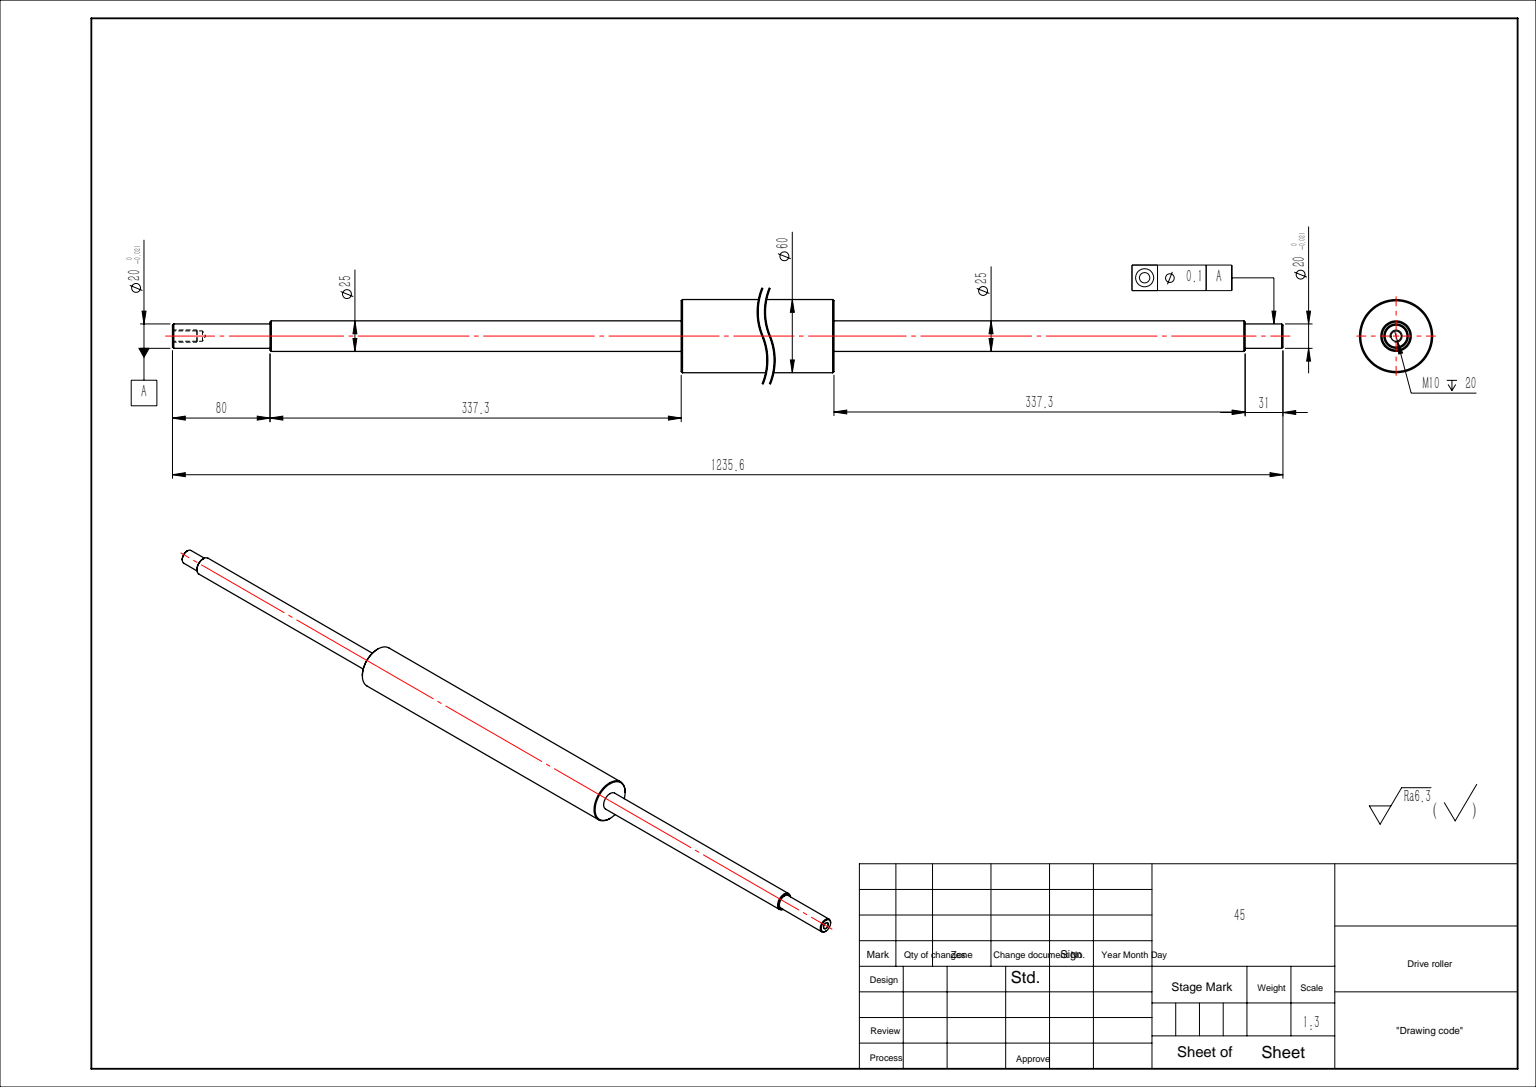
SolidWorks part; units mm, degrees
material "45"
ref_plane "前视基准面" through (0, 0, 0) normal (0, 0, 1) x (1, 0, 0)
ref_plane "上视基准面" through (0, 0, 0) normal (0, 1, 0) x (1, 0, 0)
ref_plane "右视基准面" through (0, 0, 0) normal (1, 0, 0) x (0, 0, -1)
sketch "草图1" plane through (0, 0, 0) normal (0, 0, 1) x (1, 0, 0)
  line L0 (-106.3119, -3.9821) -> (105.244, -3.9821) construction
  line L1 (0, 85.9187) -> (0, 0) construction
  line L2 (0, 0) -> (720.3653, 0) construction
  line L3 (-593.3, 0) -> (-593.3, 10)
  line L4 (-593.3, 10) -> (-562.3, 10)
  line L5 (-562.3, 10) -> (-562.3, 12.5)
  line L6 (-562.3, 12.5) -> (-225, 12.5)
  line L7 (-225, 12.5) -> (-225, 30)
  line L8 (-225, 30) -> (225, 30)
  line L9 (225, 30) -> (225, 12.5)
  line L10 (225, 12.5) -> (562.3, 12.5)
  line L11 (562.3, 12.5) -> (562.3, 10)
  line L12 (562.3, 10) -> (642.3, 10)
  line L13 (642.3, 10) -> (642.3, 0)
  line L14 (642.3, 0) -> (-593.3, 0)
  point P15 (0, 30)
  dimension "D1" = 20
  dimension "D2" = 25
  dimension "D3" = 60
  dimension "D4" = 450
  dimension "D5" = 1124.6
  dimension "D6" = 31
  dimension "D7" = 80
revolve "旋转1" add sketch "草图1" angle 360 about L14
chamfer "倒角1" distance 1 angle 45 6 edges at (642.3, 10, 0) (562.3, 12.5, 0) (225, 30, 0) (-225, 30, 0) (-562.3, 12.5, 0) (-593.3, 10, 0)
sketch "草图2" plane through (0, 0, 0) normal (1, 0, 0) x (0, 0, -1)
  circle A0 centre (0, 0) radius 30 construction
  circle A1 centre (0, 0) radius 30
hole_wizard "M10 螺纹孔1" positions "草图3" profile "草图4" tap size "M10" standard "GB"
sketch "草图3" plane through (642.3, 0, 0) normal (1, 0, 0) x (0, 0, -1)
  point P0 (0, 0)
sketch "草图4" plane through (642.3, 0, 0) normal (0, 1, 0) x (0, 0, -1)
  line L0 (0, 0) -> (0, 27.0537)
  line L1 (0, 27.0537) -> (4.25, 24.5)
  line L2 (4.25, 24.5) -> (4.25, 0)
  line L5 (4.25, 0) -> (0, 0)
  line L10 (0, 27.0537) -> (-4.25, 24.5) construction
  line L11 (0, -6.35) -> (0, 107.95) construction
  dimension "螺纹孔钻头直径" = 8.5
  dimension "螺纹孔钻头深度" = 24.5
  dimension "导头角度" = 118
cosmetic thread "孔螺蚊线1" parameters "D1"=20, "D2"=10
